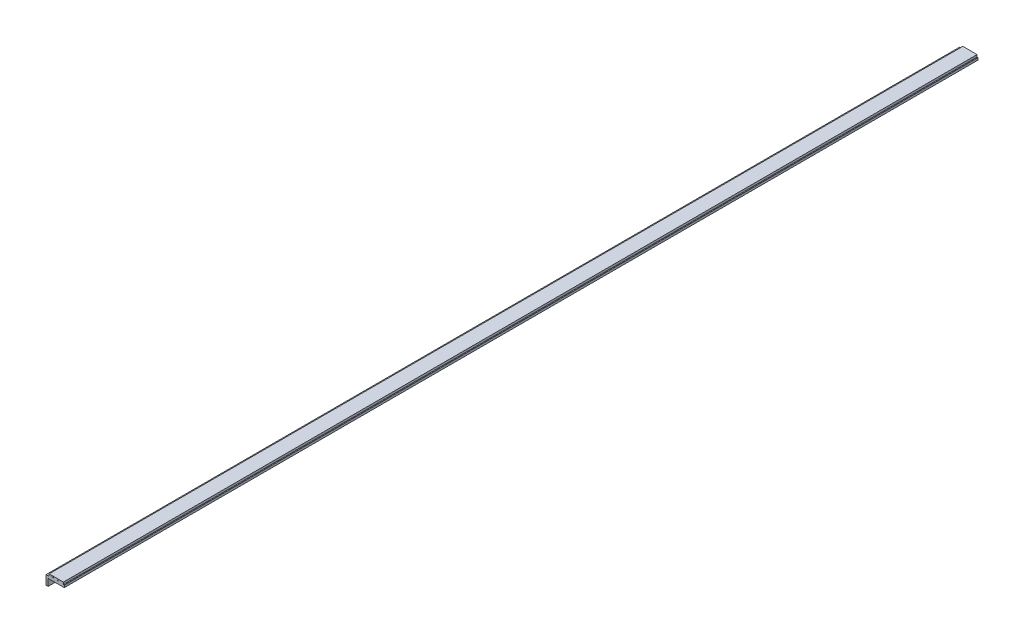
SolidWorks part; units mm, degrees
ref_plane "Front Plane" through (0, 0, 0) normal (0, 0, 1) x (1, 0, 0)
ref_plane "Top Plane" through (0, 0, 0) normal (0, 1, 0) x (1, 0, 0)
ref_plane "Right Plane" through (0, 0, 0) normal (1, 0, 0) x (0, 0, -1)
other "Configuration Table"
sketch "Sketch1" plane through (0, 0, 0) normal (0, 0, 1) x (1, 0, 0)
  line L0 (0, 0) -> (100, 0)
  line L1 (0, 0) -> (0, 100)
  line L2 (12, 12) -> (17, 12)
  line L3 (12, 12) -> (12, 100)
  line L4 (12, 100) -> (0, 100)
  line L5 (100, 12) -> (100, 0)
  line L6 (17, 12) -> (17, 24)
  line L7 (17, 24) -> (95, 24)
  line L8 (95, 24) -> (95, 12)
  line L9 (95, 12) -> (100, 12)
  line L10 (12, 12) -> (100, 12) construction
  dimension "D1" = 100
  dimension "D2" = 100
  dimension "D4" = 12
  dimension "D5" = 5
  dimension "D6" = 5
  dimension "D3" = 12
extrude "Boss-Extrude1" add sketch "Sketch1" along normal blind 5000
sketch "Sketch2" plane through (0, 0, 5000) normal (0, 0, 1) x (1, 0, 0)
  line L0 (95, 24) -> (17, 24) construction
  line L1 (21.4792, 24) -> (22.7391, 24)
  line L2 (21.4792, 24) -> (21.4792, 14.9569)
  line L3 (21.4792, 14.9569) -> (22.7391, 14.9569)
  line L4 (22.7391, 24) -> (22.7391, 14.9569)
  line L5 (21.4792, 24) -> (22.7391, 14.9569) construction
  line L6 (21.4792, 14.9569) -> (22.7391, 24) construction
  point P0 (22.1092, 19.4785)
extrude "Cut-Extrude1" cut sketch "Sketch2" against normal blind 0.2
pattern_linear "LPattern1" count 16 spacing 6 along (1, 0, 0) of "Cut-Extrude1"
ref_plane "Plane1" through (0, 0, 2500) normal (0, 0, -1) x (-1, 0, 0)
mirror "Mirror1" about plane through (0, 0, 2500) normal (0, 0, -1) of "LPattern1", "Cut-Extrude1"
sketch "Sketch3" plane through (0, 0, 5000) normal (0, 0, 1) x (1, 0, 0)
  line L1 (12, 12) -> (0, 12)
  line L2 (12, 12) -> (12, -38)
  line L3 (12, -38) -> (0, -38)
  line L4 (0, 12) -> (0, -38)
  dimension "D1" = 50
extrude "Boss-Extrude2" add sketch "Sketch3" against normal blind 5000
sketch "Sketch4" plane through (0, 0, 0) normal (0, 0, -1) x (-1, 0, 0)
  line L0 (0, 100) -> (0, -38) construction
  line L1 (-12, 100) -> (0, 100)
  line L2 (-12, 100) -> (-12, 12)
  line L3 (-12, 12) -> (0, 12)
  line L4 (0, 100) -> (0, 12)
extrude "Cut-Extrude2" cut sketch "Sketch4" against normal through all
